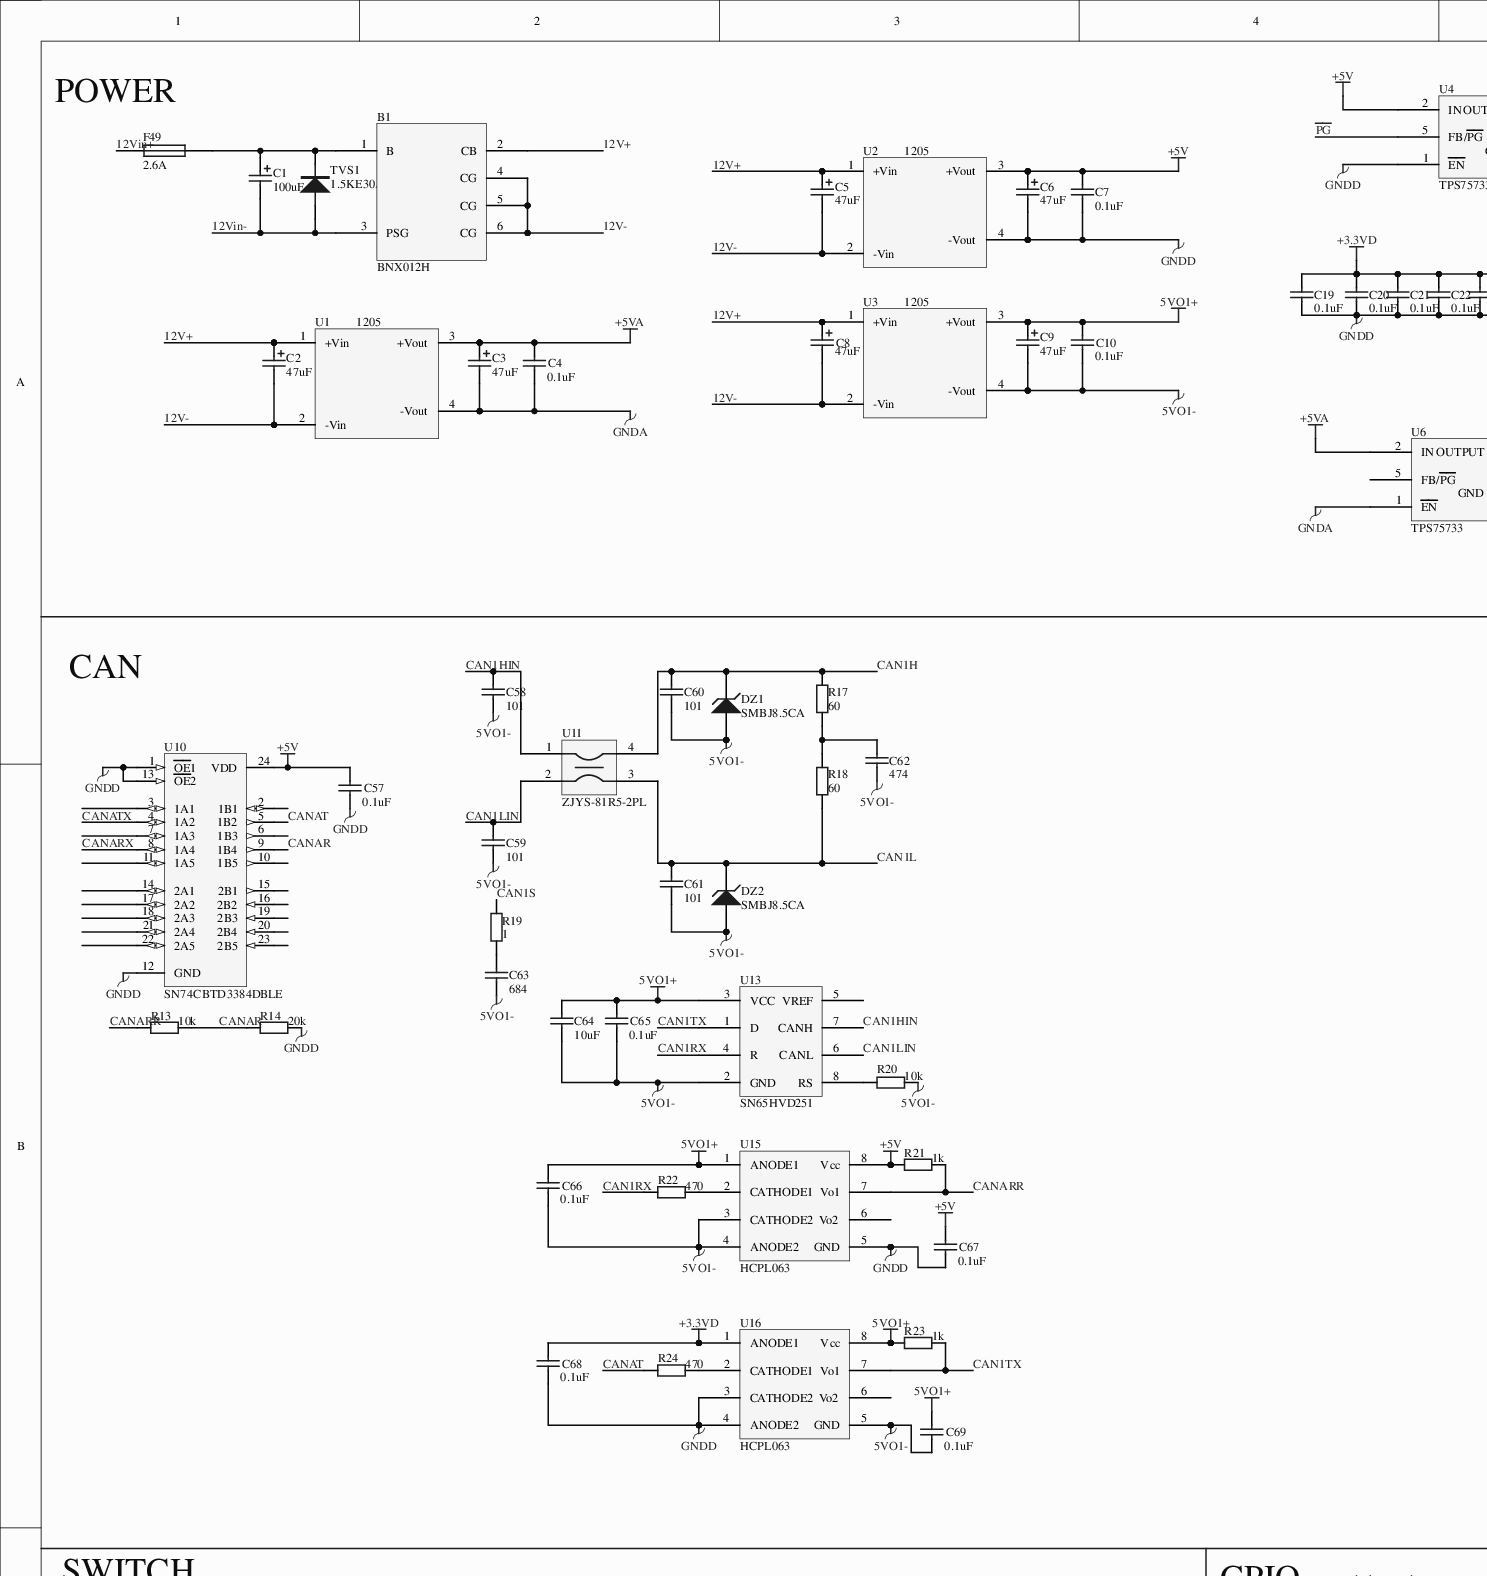
[diagram p0: MISC86180.SCHDOC, top left]
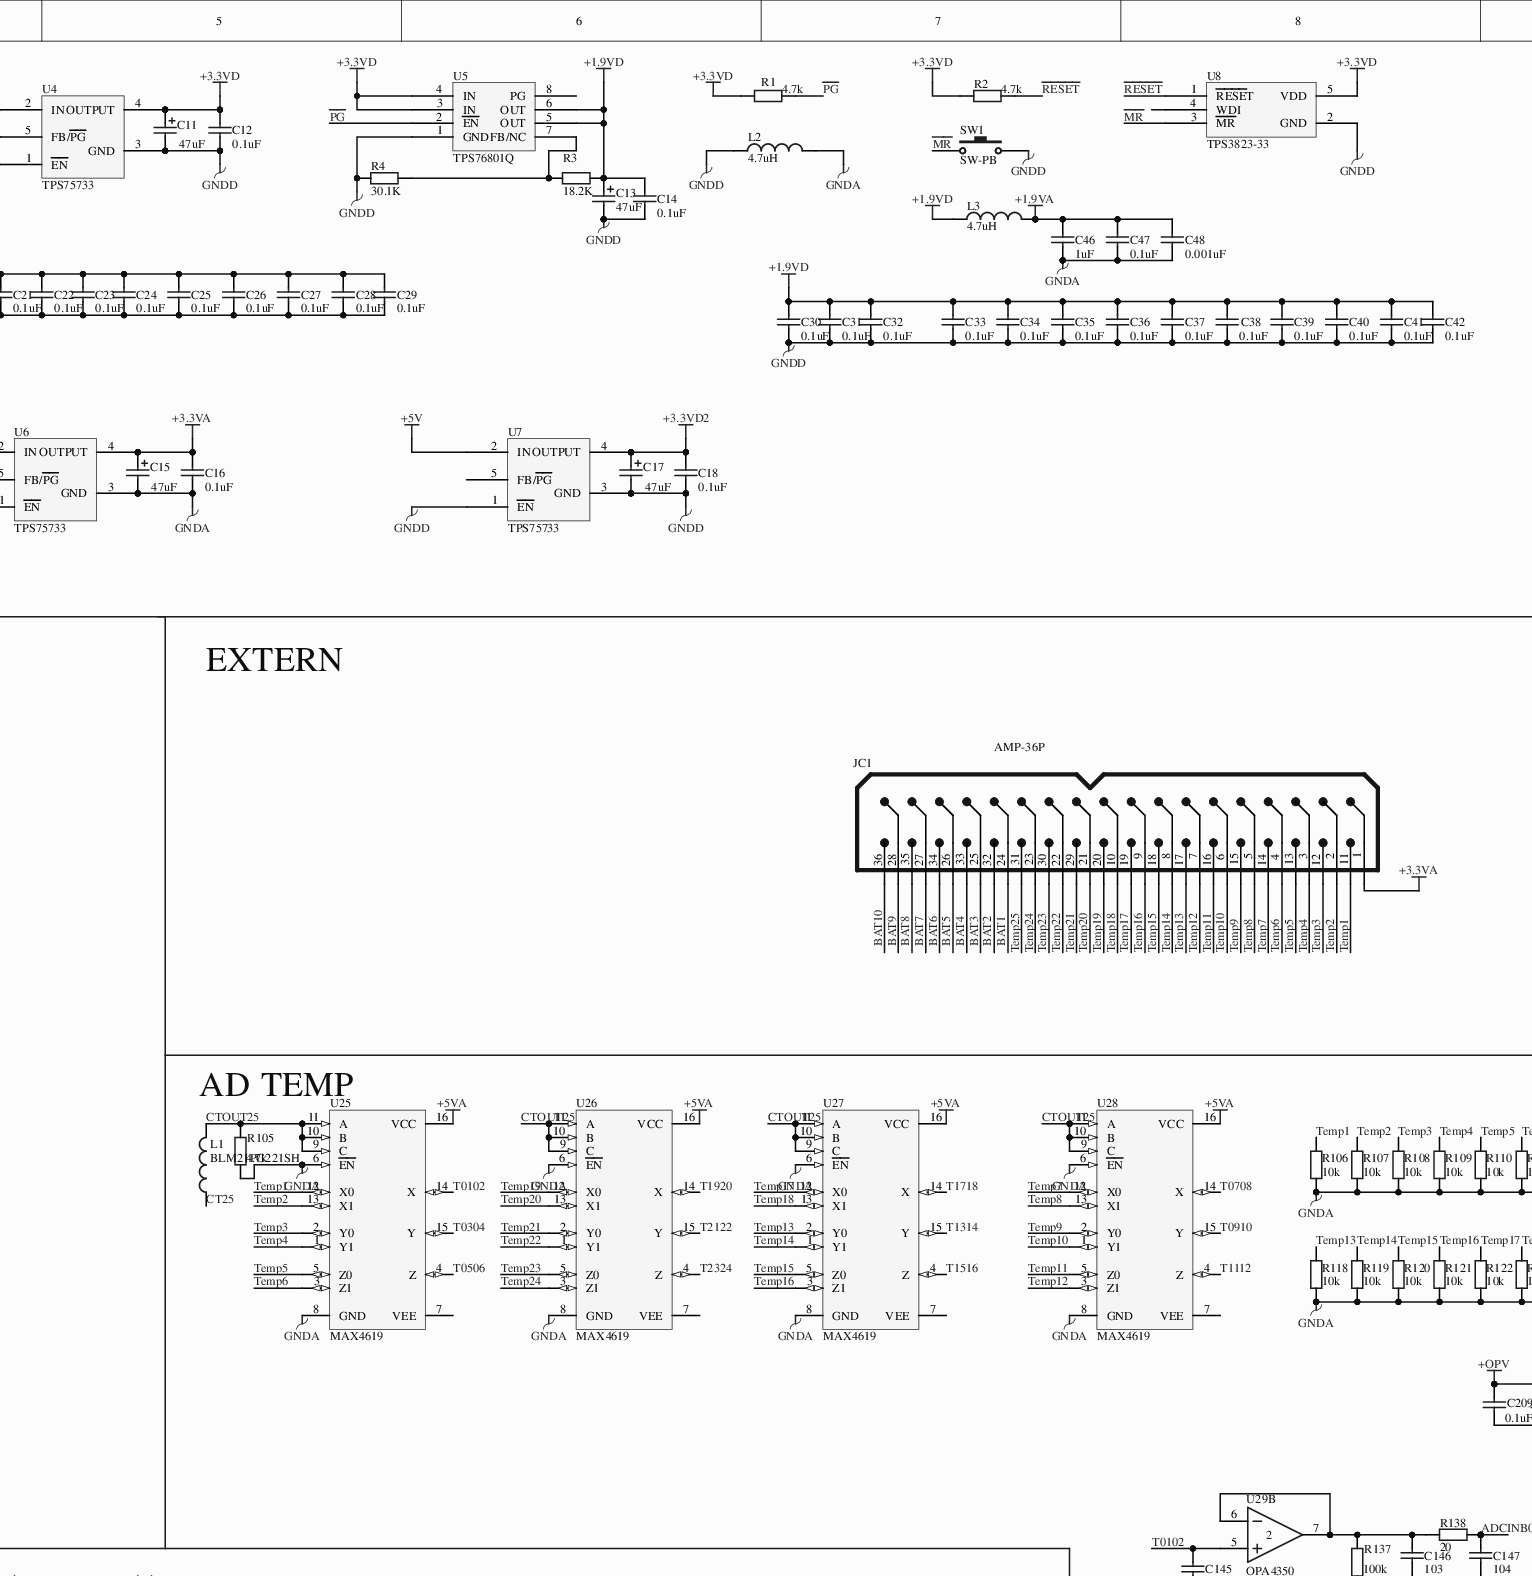
[diagram p1: MISC86180.SCHDOC, top middle]
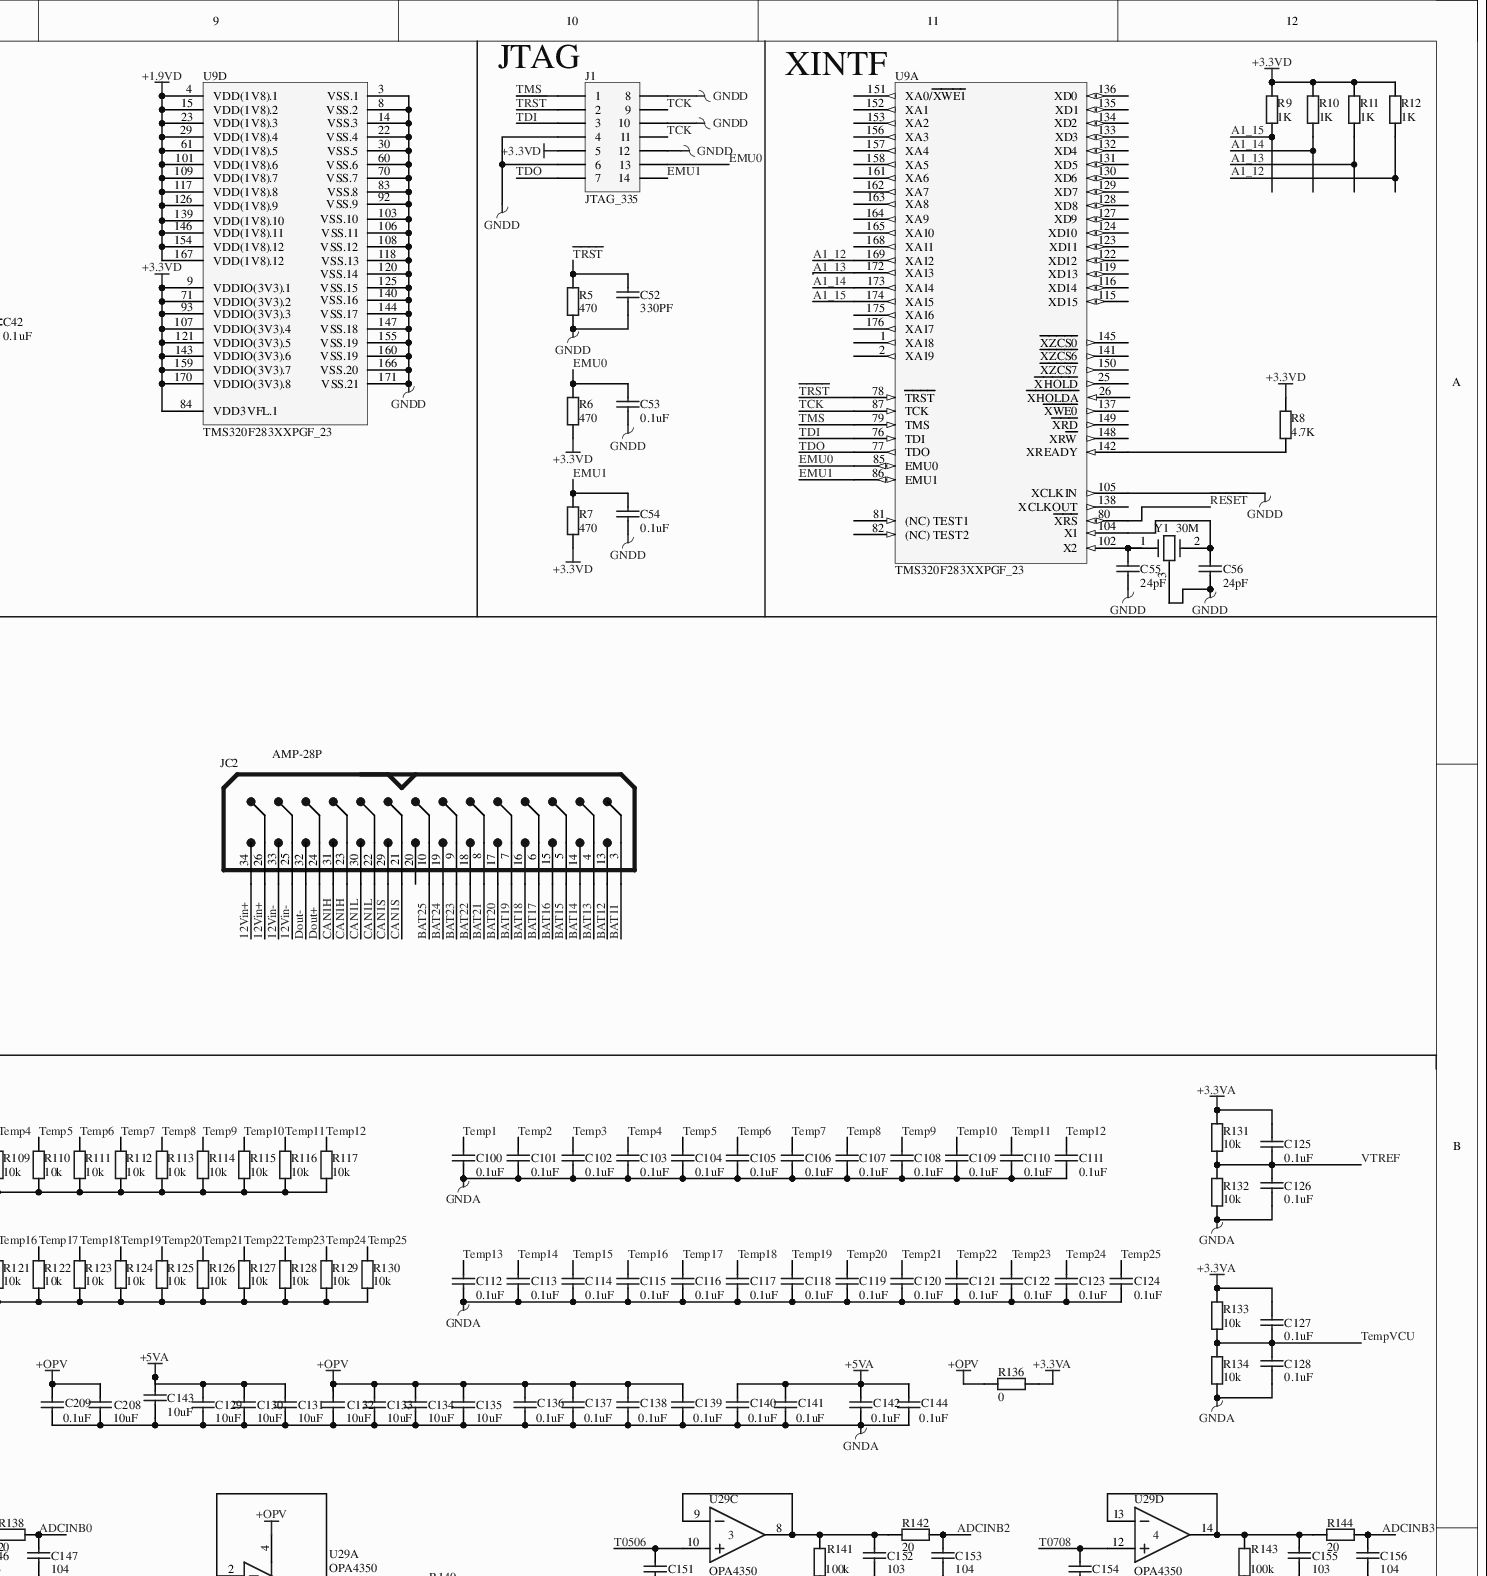
[diagram p2: MISC86180.SCHDOC, top right]
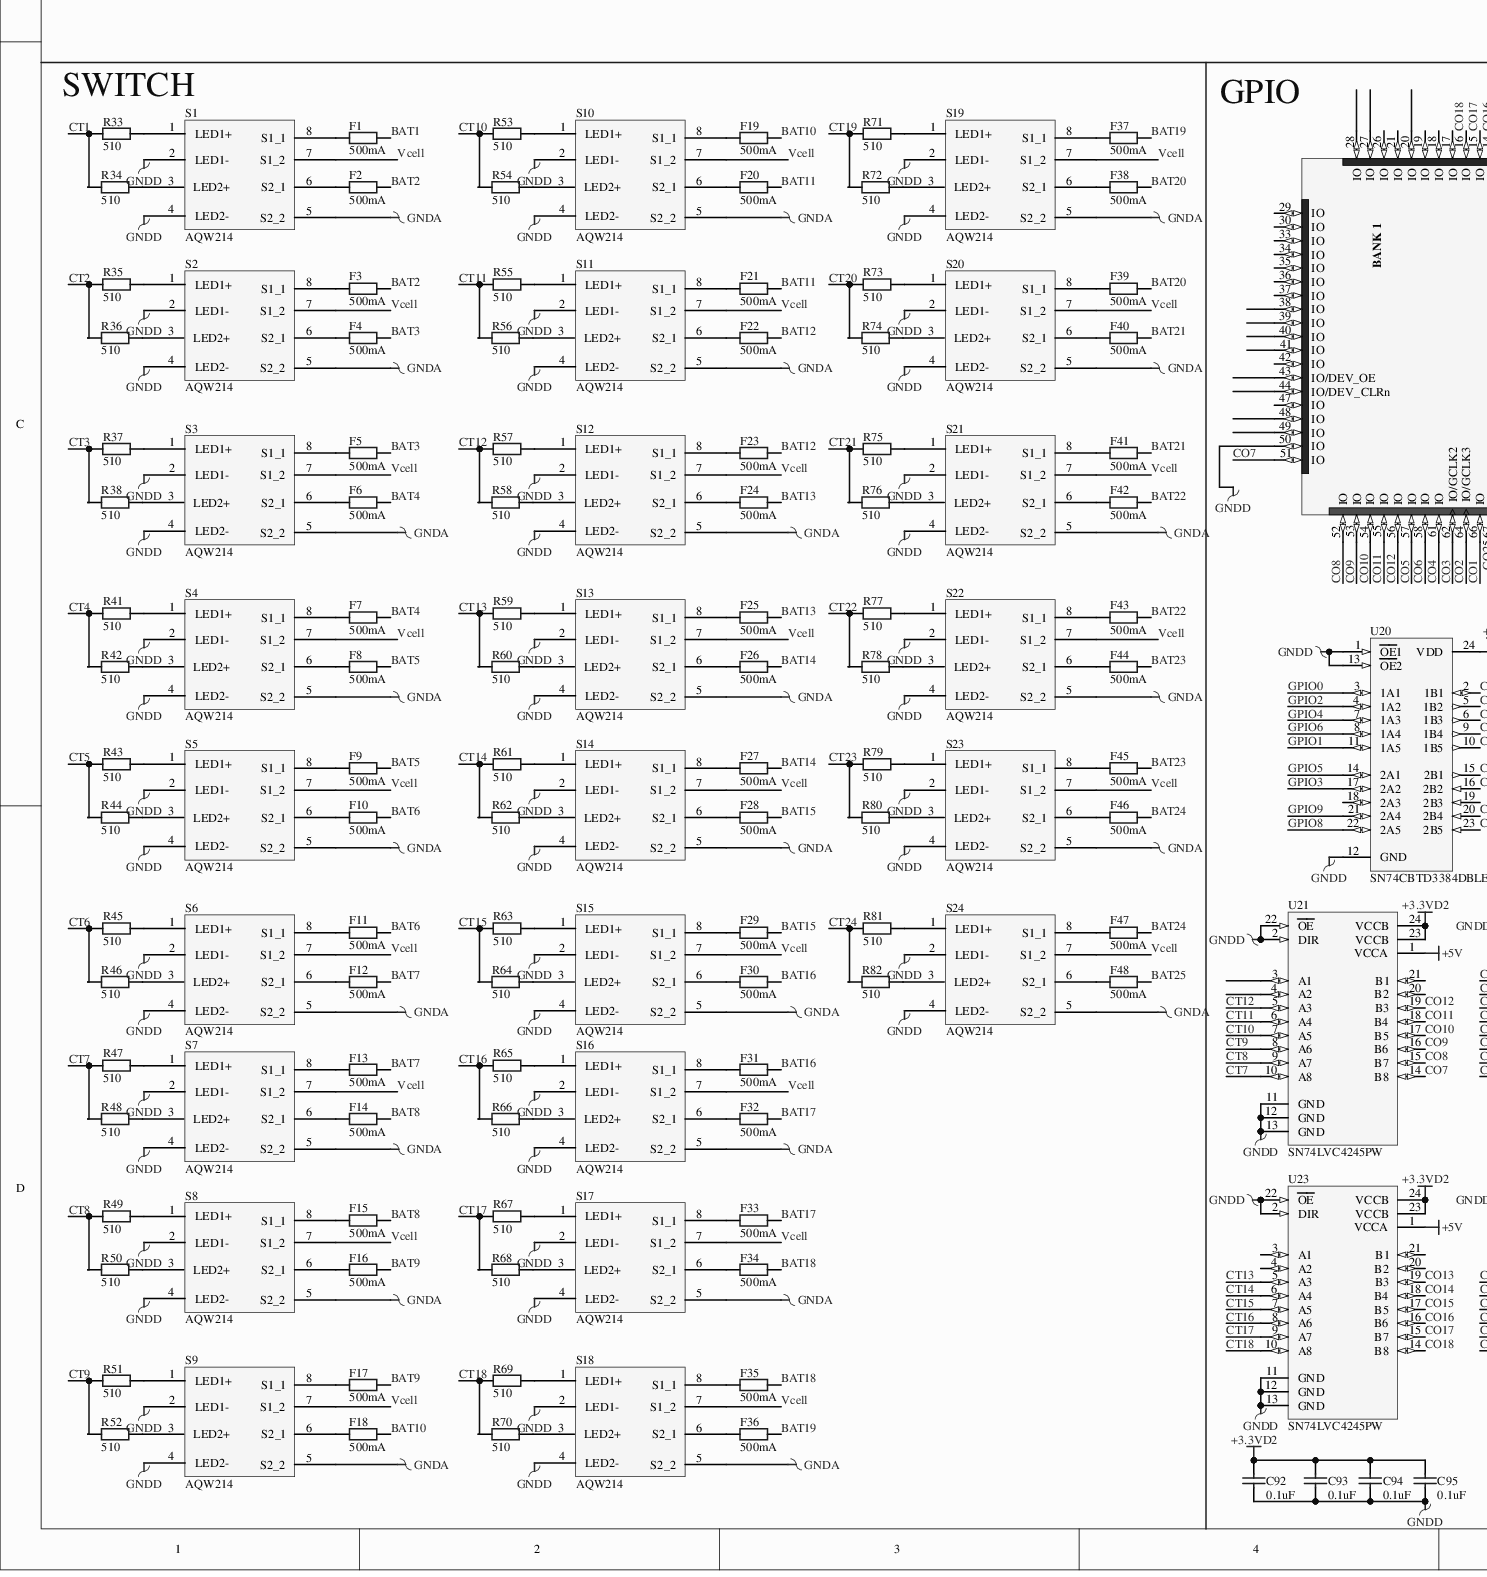
[diagram p3: MISC86180.SCHDOC, bottom left]
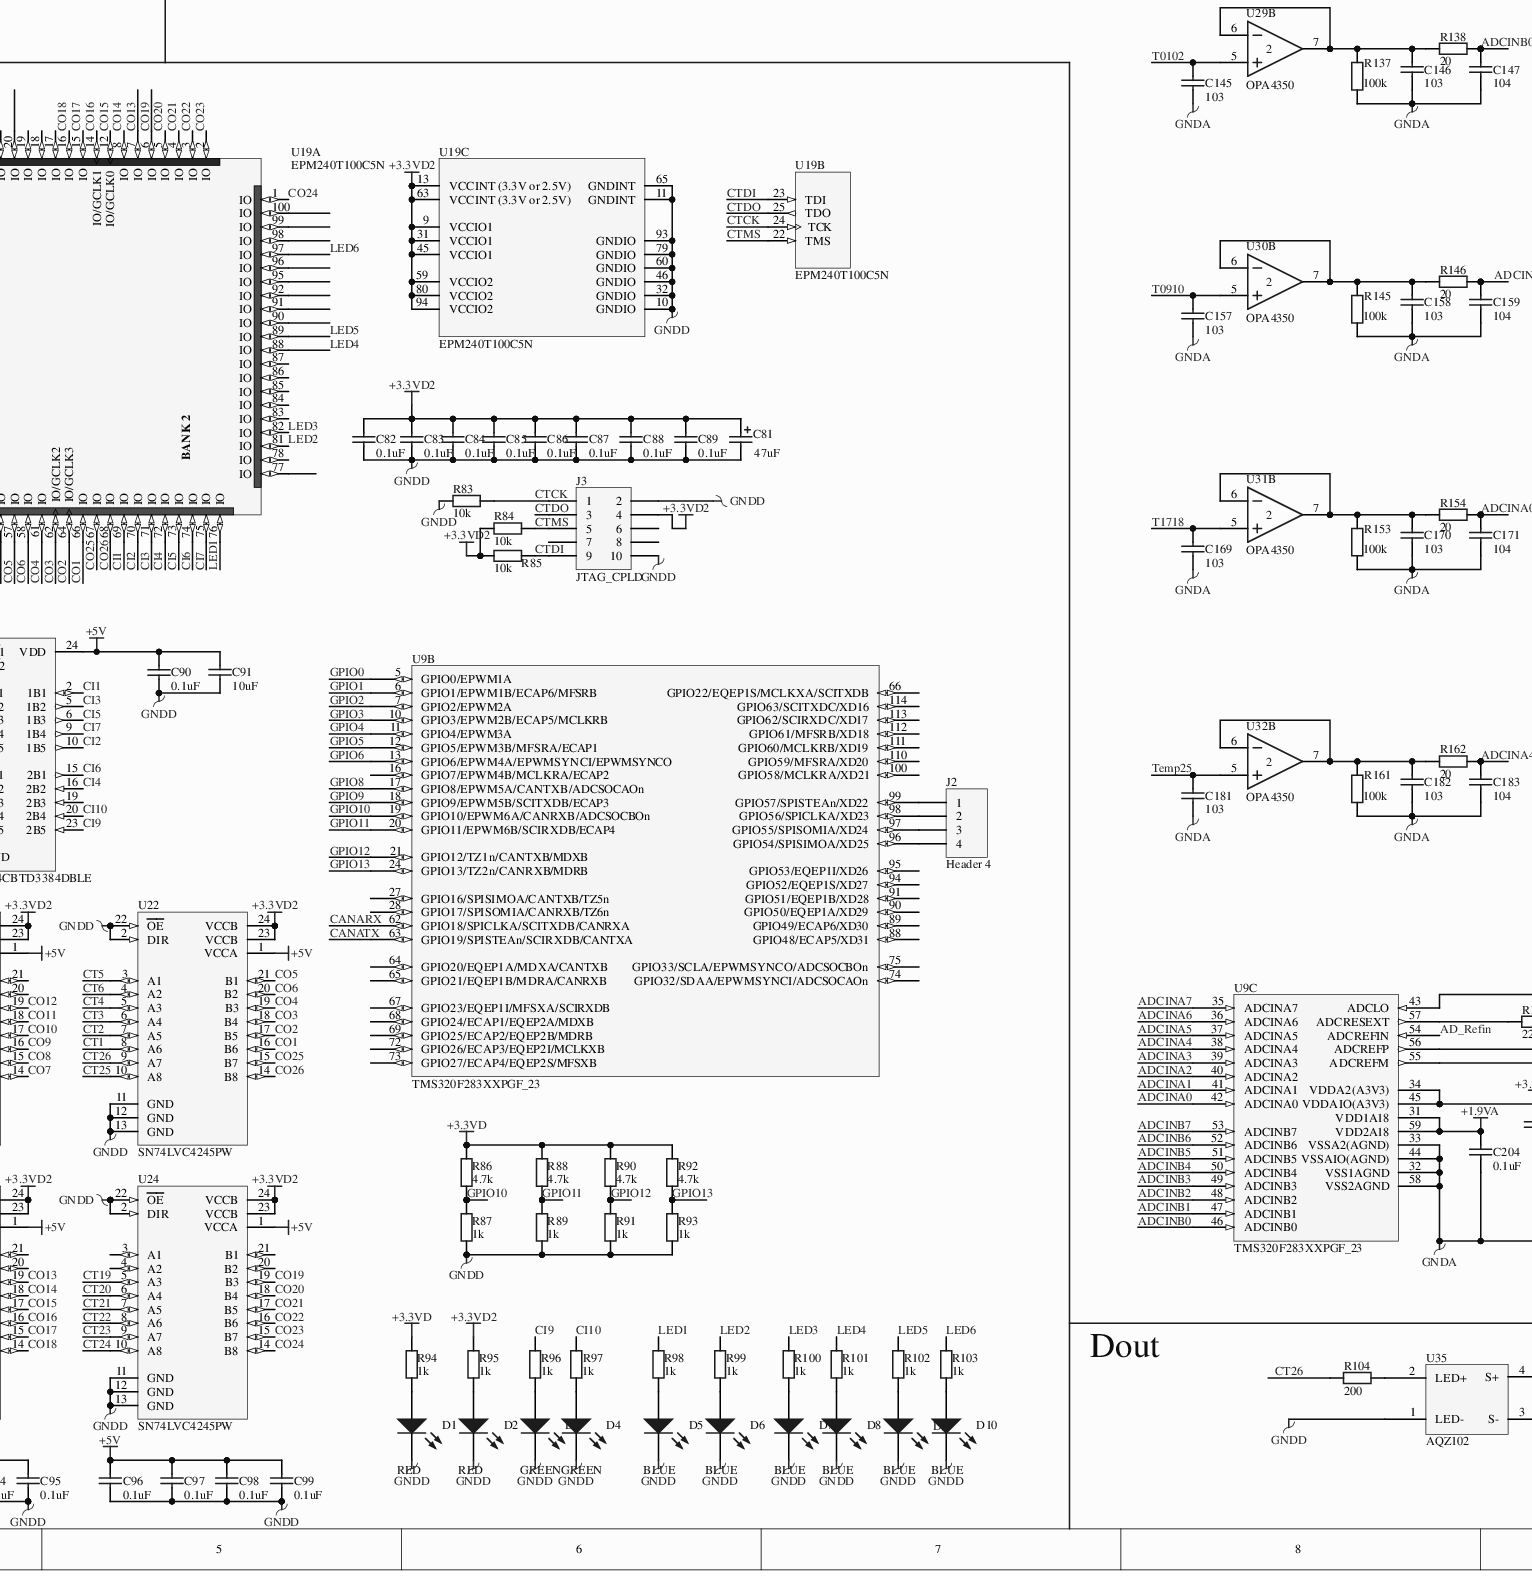
[diagram p4: MISC86180.SCHDOC, bottom middle]
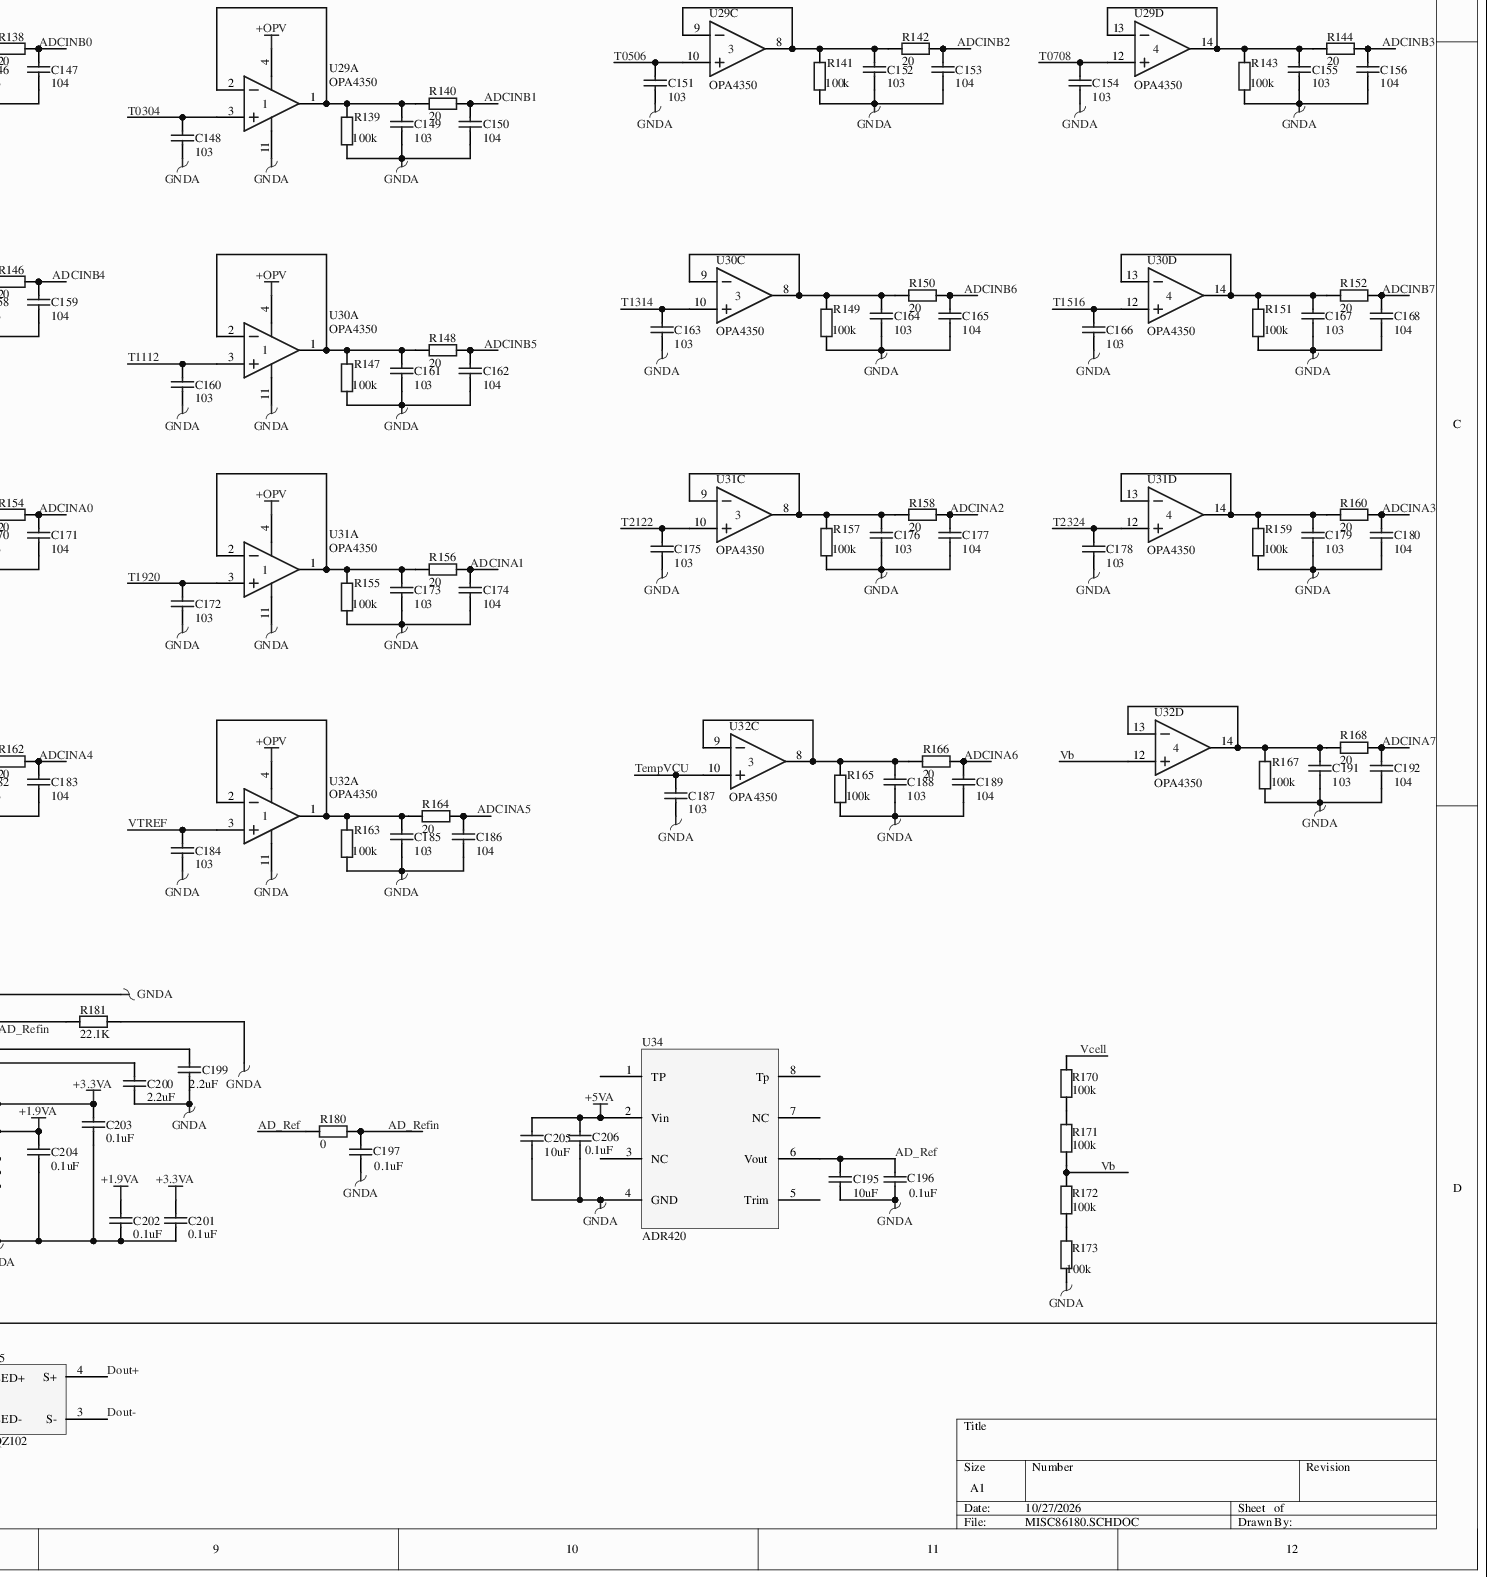
[diagram p5: MISC86180.SCHDOC, bottom right]
# Altium project MISC86180-9.PrjPCB (part 1 of 3)
1 sheet, 475 parts. Net scope: global (net labels, ports and power ports of the same name join across sheets).
Board file: MISC86180.PCBDOC